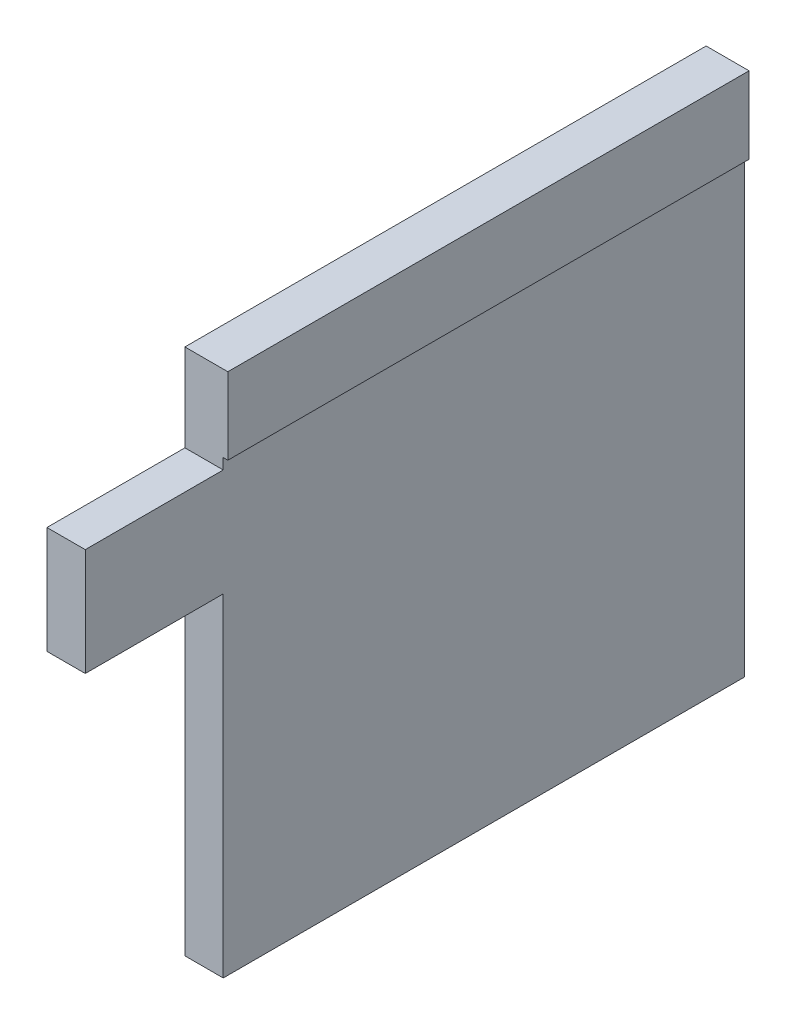
SolidWorks part; units mm, degrees
ref_plane "前视基准面" through (0, 0, 0) normal (0, 0, 1) x (1, 0, 0)
ref_plane "上视基准面" through (0, 0, 0) normal (0, 1, 0) x (1, 0, 0)
ref_plane "右视基准面" through (0, 0, 0) normal (1, 0, 0) x (0, 0, -1)
sketch "草图1" plane through (0, 0, 0) normal (0, 0, 1) x (1, 0, 0)
  line L0 (0, 0) -> (0, 172)
  line L1 (0, 172) -> (14, 172)
  line L2 (14, 172) -> (14, 147)
  line L3 (14, 147) -> (12.5, 147)
  line L4 (12.5, 147) -> (12.5, 0)
  line L5 (12.5, 0) -> (0, 0)
  dimension "D1" = 147
  dimension "D2" = 14
  dimension "D3" = 25
  dimension "D4" = 1.5
extrude "凸台-拉伸1" add sketch "草图1" along normal mid plane 170
sketch "草图2" plane through (0, 0, 0) normal (-1, 0, 0) x (0, 0, 1)
  line L0 (85, 0) -> (-85, 0) construction
  line L1 (-85, 172) -> (-85, 0) construction
  circle A0 centre (-73, 13) radius 6
  dimension "D1" = 12
  dimension "D2" = 13
  dimension "D3" = 12
extrude "切除-拉伸1" [suppressed] cut sketch "草图2" against normal blind 7
hole_wizard "M10x1.25 螺纹孔1" positions "3D草图1" profile "草图3" tap size "M10x1.25" standard "GB"
sketch3d "3D草图1" [suppressed]
  circle A0 centre (0, 13, -73) radius 6 construction
  point P0 (7, 13, -73)
  point P5 (-6, 13, -73)
sketch "草图3" plane through (7, 13, -73) normal (0, 1, 0) x (0, 0, 1)
  line L0 (0, 0) -> (0, 5.5)
  line L1 (0, 5.5) -> (4.4, 5.5)
  line L2 (4.4, 5.5) -> (4.4, 0)
  line L5 (4.4, 0) -> (0, 0)
  line L11 (0, -6.35) -> (0, 107.95) construction
  dimension "通孔螺纹孔钻头直径" = 8.8
  dimension "通孔螺纹孔钻头深度" = 5.5
cosmetic thread "孔螺蚊线1" parameters "D2"=10
sketch "草图4" plane through (0, 0, 85) normal (0, 0, -1) x (-1, 0, 0)
  line L1 (-12.5, 143.5) -> (0, 143.5)
  line L2 (-12.5, 143.5) -> (-12.5, 108.5)
  line L3 (-12.5, 108.5) -> (0, 108.5)
  line L4 (0, 143.5) -> (0, 108.5)
  line L5 (0, 172) -> (0, 0) construction
  line L6 (-14, 172) -> (0, 172) construction
  line L7 (-12.5, 0) -> (-12.5, 147) construction
  point P4 (0, 0)
  point P10 (0, 0)
  dimension "D1" = 28.5
  dimension "D2" = 35
extrude "凸台-拉伸2" add sketch "草图4" against normal blind 45
